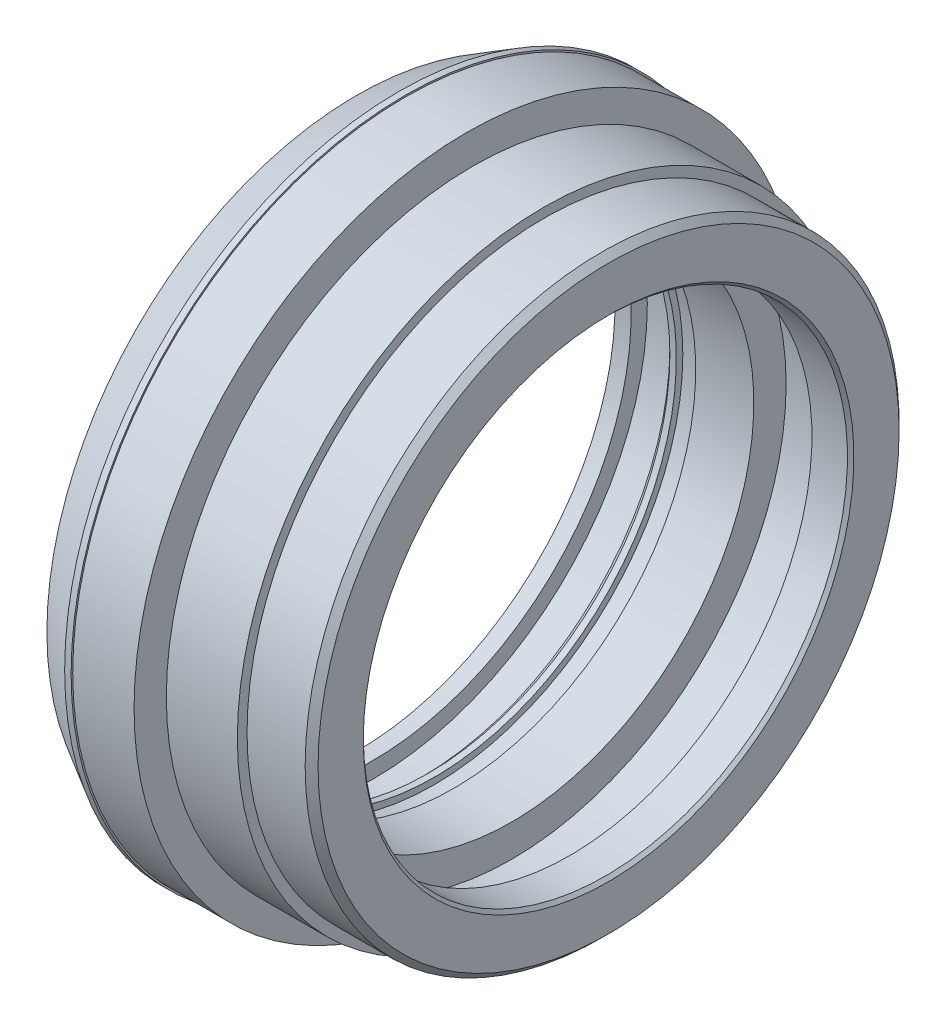
SolidWorks part; units mm, degrees
ref_plane "前视基准面" through (0, 0, 0) normal (0, 0, 1) x (1, 0, 0)
ref_plane "上视基准面" through (0, 0, 0) normal (0, 1, 0) x (1, 0, 0)
ref_plane "右视基准面" through (0, 0, 0) normal (1, 0, 0) x (0, 0, -1)
sketch "草图1" plane through (0, 0, 0) normal (0, 1, 0) x (1, 0, 0)
  line L0 (-85.1032, 0) -> (68.0547, 0) construction
  line L1 (5.0349, 40) -> (7.5349, 40)
  line L2 (7.5349, 40) -> (7.5349, 42.5)
  line L3 (7.5349, 42.5) -> (15.0349, 42.5)
  line L4 (15.0349, 42.5) -> (15.0349, 37.5)
  line L5 (15.0349, 37.5) -> (17.0349, 37.5)
  line L6 (17.0349, 37.5) -> (17.0349, 38.5)
  line L7 (17.0349, 38.5) -> (20.0349, 38.5)
  line L8 (20.0349, 38.5) -> (20.0349, 37.5)
  line L9 (20.0349, 37.5) -> (29.0349, 37.5)
  line L10 (29.0349, 37.5) -> (29.0349, 42.5)
  line L11 (29.0349, 42.5) -> (38.0349, 42.5)
  line L12 (38.0349, 42.5) -> (38.0349, 37.5)
  line L13 (38.0349, 37.5) -> (44.0349, 37.5)
  line L14 (44.0349, 37.5) -> (44.0349, 46)
  line L15 (44.0349, 46) -> (34.0349, 46)
  line L16 (34.0349, 46) -> (34.0349, 47.5)
  line L17 (34.0349, 47.5) -> (23.0349, 47.5)
  line L18 (23.0349, 47.5) -> (23.0349, 46)
  line L19 (23.0349, 46) -> (22.0349, 46)
  line L20 (5.0349, 40) -> (5.0349, 48)
  line L21 (5.0349, 48) -> (11.5349, 51.75)
  line L22 (22.0349, 46) -> (22.0349, 51.5)
  line L23 (22.0349, 51.5) -> (12.5349, 51.5)
  line L24 (12.5349, 51.5) -> (12.5349, 51.75)
  line L25 (12.5349, 51.75) -> (11.5349, 51.75)
  dimension "D1" = 40
  dimension "D2" = 2.5
  dimension "D3" = 2.5
  dimension "D4" = 7.5
  dimension "D5" = 5
  dimension "D6" = 2
  dimension "D7" = 1
  dimension "D8" = 1
  dimension "D9" = 3
  dimension "D10" = 5
  dimension "D11" = 5
  dimension "D12" = 9
  dimension "D13" = 6
  dimension "D14" = 8.5
  dimension "D15" = 10
  dimension "D16" = 11
  dimension "D17" = 1
  dimension "D18" = 1.5
  dimension "D19" = 1.5
  dimension "D20" = 5.5
  dimension "D21" = 9.5
  dimension "D22" = 0.25
  dimension "D23" = 1
  dimension "D24" = 9
  dimension "D25" = 8
revolve "旋转1" add sketch "草图1" angle 360 about L0
cosmetic thread "装饰螺纹线1" parameters "D2"=57.505
chamfer "倒角1" distance 1 angle 45 1 edges at (44.0349, 0, 46)
chamfer "倒角2" distance 0.5 angle 45 1 edges at (44.0349, 0, 37.5)
chamfer "倒角3" distance 1 angle 45 1 edges at (15.0349, 0, 37.5)
